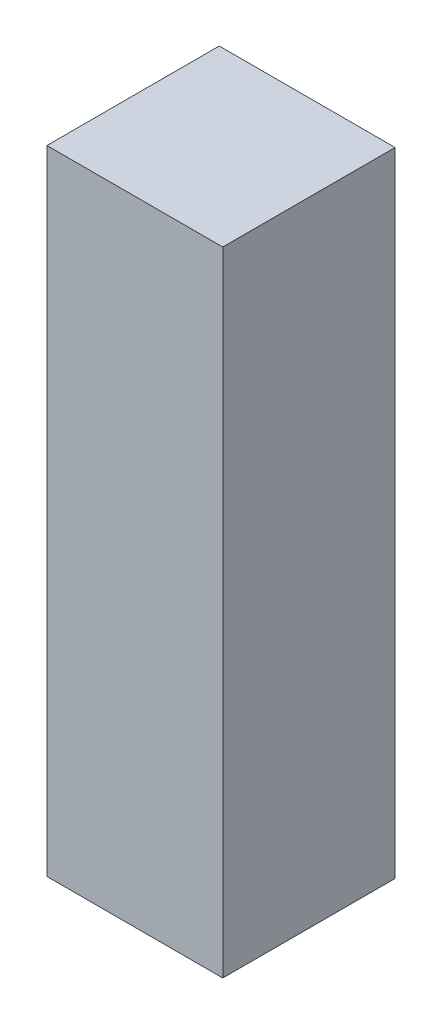
SolidWorks part; units mm, degrees
ref_plane "前视基准面" through (0, 0, 0) normal (0, 0, 1) x (1, 0, 0)
ref_plane "上视基准面" through (0, 0, 0) normal (0, 1, 0) x (1, 0, 0)
ref_plane "右视基准面" through (0, 0, 0) normal (1, 0, 0) x (0, 0, -1)
sketch "草图1" plane through (0, 0, 0) normal (0, 0, 1) x (1, 0, 0)
  line L1 (0, 45) -> (25, 45)
  line L2 (0, 45) -> (0, -45)
  line L3 (0, -45) -> (25, -45)
  line L4 (25, 45) -> (25, -45)
  dimension "D1" = 90
  dimension "D2" = 25
extrude "凸台-拉伸1" add sketch "草图1" along normal blind 24.5
